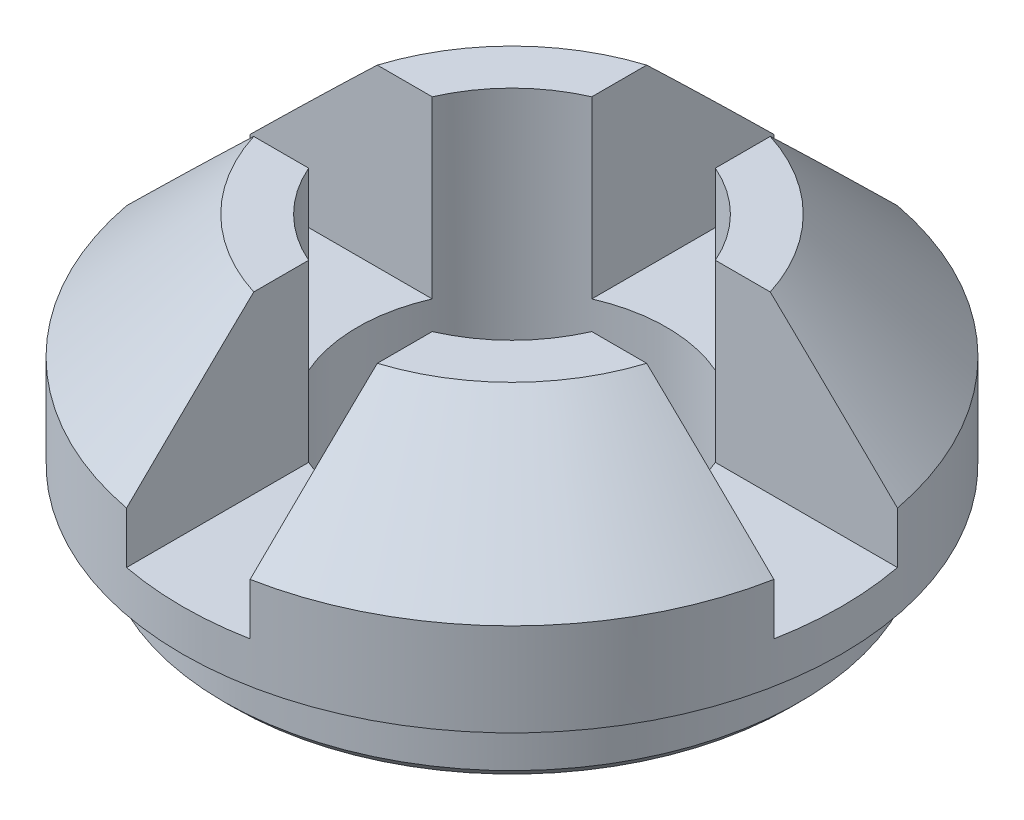
SolidWorks part; units mm, degrees
ref_plane "Front Plane" through (0, 0, 0) normal (0, 0, 1) x (1, 0, 0)
ref_plane "Top Plane" through (0, 0, 0) normal (0, 1, 0) x (1, 0, 0)
ref_plane "Right Plane" through (0, 0, 0) normal (1, 0, 0) x (0, 0, -1)
other "Configuration Table"
sketch "Sketch1" plane through (0, 0, 0) normal (0, 0, 1) x (1, 0, 0)
  line L0 (0, 0) -> (0, 21.5752) construction
  line L1 (0, 0) -> (-14, 0)
  line L2 (-14, 0) -> (-14, 3.5)
  line L3 (-14, 3.5) -> (-16, 3.5)
  line L4 (-16, 3.5) -> (-16, 8)
  line L5 (0, 0) -> (0, 14)
  line L7 (-16, 8) -> (-10, 14)
  line L8 (-10, 14) -> (0, 14)
  dimension "D1" = 14
  dimension "D2" = 3.5
  dimension "D3" = 4.5
  dimension "D4" = 45
  dimension "D5" = 28
  dimension "D6" = 20
revolve "Revolve1" add sketch "Sketch1" angle 360 about L0
sketch "Sketch2" plane through (0, 14, 0) normal (0, 1, 0) x (1, 0, 0)
  circle A0 centre (0, 0) radius 7.5
  dimension "D1" = 15
extrude "Cut-Extrude1" cut sketch "Sketch2" against normal blind 31
sketch "Sketch3" plane through (0, 14, 0) normal (0, 1, 0) x (1, 0, 0)
  line L1 (-20.34, 3) -> (20.34, 3)
  line L2 (-20.34, 3) -> (-20.34, -3)
  line L3 (-20.34, -3) -> (20.34, -3)
  line L4 (20.34, 3) -> (20.34, -3)
  line L5 (-20.34, 3) -> (20.34, -3) construction
  line L6 (-20.34, -3) -> (20.34, 3) construction
  point P0 (0, 0)
  dimension "D1" = 6
extrude "Cut-Extrude2" cut sketch "Sketch3" against normal blind 8.5
pattern_circular "CirPattern1" count 4 over 360 about axis through (0, -17, 0) along (0, 1, 0) of "Cut-Extrude2"
chamfer "Chamfer1" distance 0.5 angle 45 1 edges at (0, 0, -14)
chamfer "Chamfer2" distance 0.5 angle 45 1 edges at (0, 0, 7.5)
